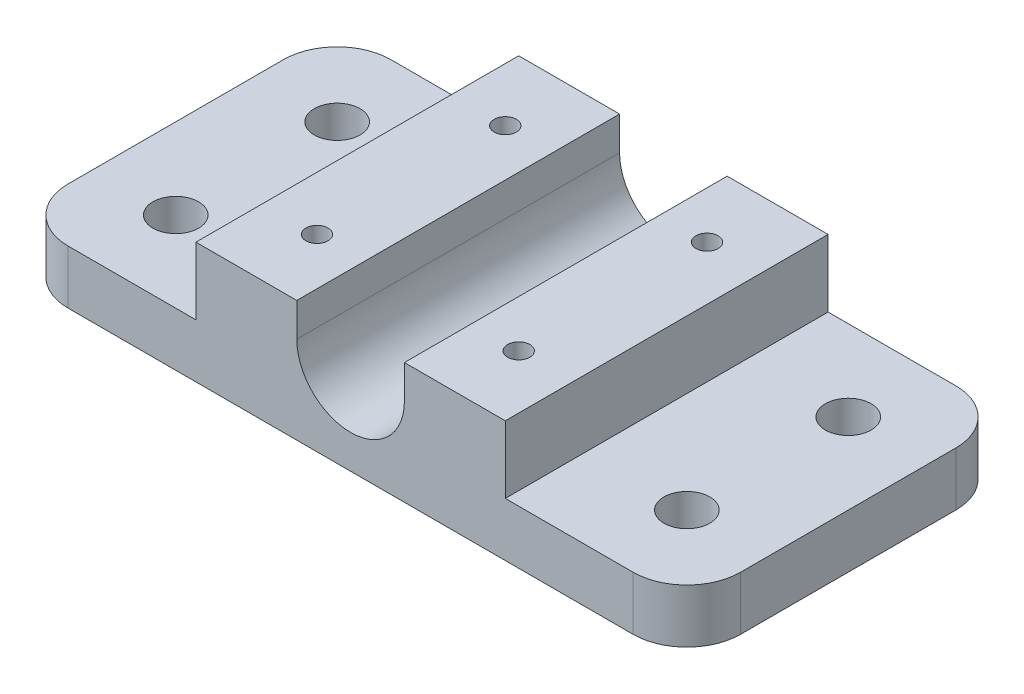
from build123d import *

# Parameters (mm, degrees)
SKETCH1_W             = 100
SKETCH1_H             = 48
BOSS_EXTRUDE1_DEPTH   = 8
SKETCH2_W             = 46
SKETCH2_H             = 48
BOSS_EXTRUDE2_DEPTH   = 10
CUT_EXTRUDE1_DEPTH    = 72.61005516
FILLET1_R             = 8
M4_TAPPED_HOLE1_D     = 3.3
M4_TAPPED_HOLE1_DEPTH = 10
M4_TAPPED_HOLE1_TIP   = 0.991420021
M8_TAPPED_HOLE1_D     = 6.8


with BuildPart() as part:
    # Sketch1 → Boss-Extrude1 (new body)
    with BuildSketch(Plane(origin=(0, 0, 0), x_dir=(1, 0, 0), z_dir=(0, 1, 0))):
        Rectangle(SKETCH1_W, SKETCH1_H)
    extrude(amount=BOSS_EXTRUDE1_DEPTH)

    # Sketch2 → Boss-Extrude2 (add)
    with BuildSketch(Plane(origin=(0, 8, 0), x_dir=(1, 0, 0), z_dir=(0, 1, 0))):
        Rectangle(SKETCH2_W, SKETCH2_H)
    extrude(amount=BOSS_EXTRUDE2_DEPTH)

    # Sketch3 → Cut-Extrude1 (cut, through all)
    with BuildSketch(Plane.XY.offset(24)):
        with BuildLine():
            Line((-8, 13), (-8, 18))
            Line((-8, 18), (8, 18))
            Line((8, 18), (8, 13))
            ThreePointArc((8, 13), (0, 5), (-8, 13))
        make_face()
    extrude(amount=-CUT_EXTRUDE1_DEPTH, mode=Mode.SUBTRACT)

    # Fillet1
    fillet1_edges = [part.edges().sort_by_distance(p)[0] for p in [
        (50, 4, 24),
        (-50, 4, 24),
        (-50, 4, -24),
        (50, 4, -24),
    ]]
    fillet(fillet1_edges, radius=FILLET1_R)

    # M4 Tapped Hole1
    with Locations(Plane(origin=(0, 18, 0), x_dir=(1, 0, 0), z_dir=(0, 1, 0))):
        with Locations((-15, 14), (-15, -14), (15, -14), (15, 14)):
            Hole(M4_TAPPED_HOLE1_D / 2, depth=M4_TAPPED_HOLE1_DEPTH)
            with Locations((0, 0, -(M4_TAPPED_HOLE1_DEPTH + M4_TAPPED_HOLE1_TIP / 2))):  # 118° drill point
                Cone(0, M4_TAPPED_HOLE1_D / 2, M4_TAPPED_HOLE1_TIP, mode=Mode.SUBTRACT)

    # M8 Tapped Hole1 (through all)
    with Locations(Plane(origin=(0, 8, 0), x_dir=(1, 0, 0), z_dir=(0, 1, 0))):
        with Locations((-38, 12), (-38, -12), (38, -12), (38, 12)):
            Hole(M8_TAPPED_HOLE1_D / 2)


solid = part.part
